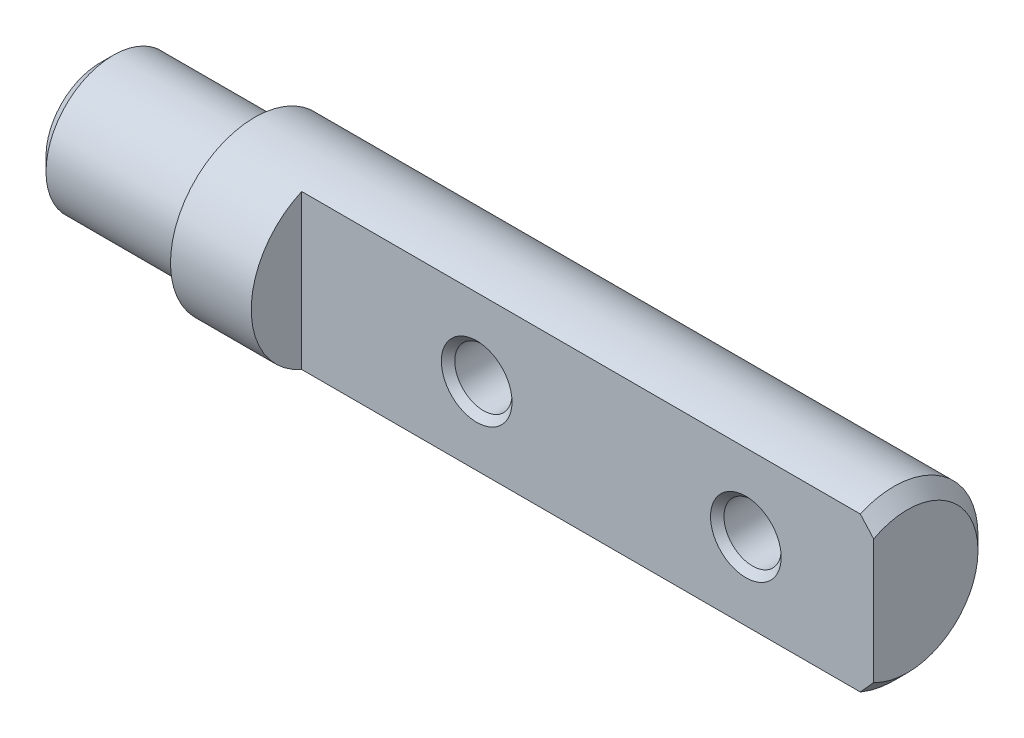
from build123d import *

# Parameters (mm, degrees)
CHAMFER_1_SIZE           = 2
CUT_EXTRUDE_1_DEPTH      = 31
CUT_EXTRUDE_1_DEPTH_BACK = 20
SKETCH_2_W               = 91.624519514
SKETCH_2_H               = 25.767863676
HOLE_WIZARD_M10_1_D      = 8.5
HOLE_WIZARD_M10_1_DEPTH  = 27.5
HOLE_WIZARD_M10_1_TIP    = 2.553657631
CHAMFER_3_SIZE           = 1


with BuildPart() as part:
    # 草图1 → 旋转2 (revolve)
    with BuildSketch(Plane.XY):
        Polygon((0, 0), (0, 10), (23, 10), (23, 12.5), (120, 12.5), (120, 0), align=None)
    revolve(axis=Axis((120, 0, 0), (-1, 0, 0)))

    # 倒角1
    chamfer_1_edges = [part.edges().sort_by_distance(p)[0] for p in [
        (120, -12.5, 0),
        (0, -10, 0),
    ]]
    chamfer(chamfer_1_edges, length=CHAMFER_1_SIZE)

    # 草图2 → 切除-拉伸1 (cut, two sides: drawn at the far end of the back side and taken through both)
    with BuildSketch(Plane(origin=(0, 0, 0), x_dir=(1, 0, 0), z_dir=(0, 1, 0)).offset(-CUT_EXTRUDE_1_DEPTH_BACK)):
        with Locations((80.812259757, -17.883931838)):
            Rectangle(SKETCH_2_W, SKETCH_2_H)
    extrude(amount=CUT_EXTRUDE_1_DEPTH + CUT_EXTRUDE_1_DEPTH_BACK, mode=Mode.SUBTRACT)

    # M10 螺纹孔1
    with Locations(Plane.XY.offset(5)):
        with Locations((61, 0), (101, 0)):
            Hole(HOLE_WIZARD_M10_1_D / 2, depth=HOLE_WIZARD_M10_1_DEPTH)
            with Locations((0, 0, -(HOLE_WIZARD_M10_1_DEPTH + HOLE_WIZARD_M10_1_TIP / 2))):  # 118° drill point
                Cone(0, HOLE_WIZARD_M10_1_D / 2, HOLE_WIZARD_M10_1_TIP, mode=Mode.SUBTRACT)

    # 倒角3
    chamfer_3_edges = [part.edges().sort_by_distance(p)[0] for p in [
        (105.25, 0, 5),
        (65.25, 0, 5),
    ]]
    chamfer(chamfer_3_edges, length=CHAMFER_3_SIZE)


solid = part.part
